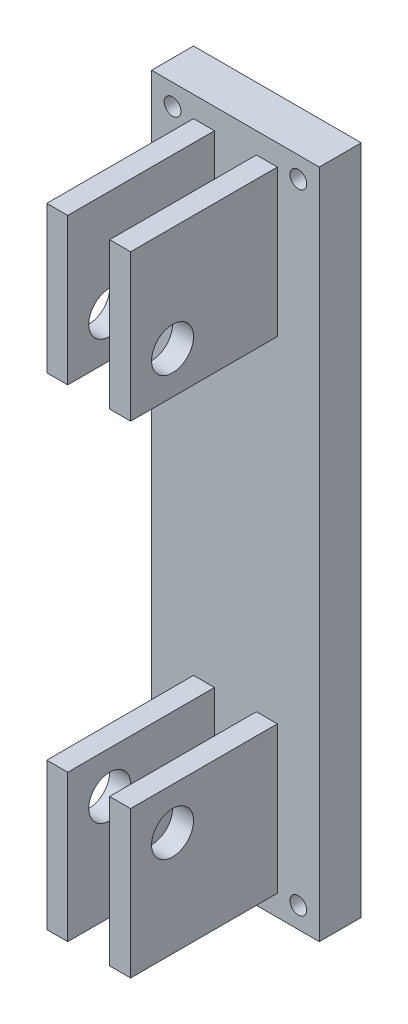
SolidWorks part; units mm, degrees
ref_plane "Front Plane" through (0, 0, 0) normal (0, 0, 1) x (1, 0, 0)
ref_plane "Top Plane" through (0, 0, 0) normal (0, 1, 0) x (1, 0, 0)
ref_plane "Right Plane" through (0, 0, 0) normal (1, 0, 0) x (0, 0, -1)
sketch "Sketch1" plane through (0, 0, 0) normal (0, 0, 1) x (1, 0, 0)
  line L1 (2, -8) -> (-2, -8)
  line L2 (2, -8) -> (2, 8)
  line L3 (2, 8) -> (-2, 8)
  line L4 (-2, -8) -> (-2, 8)
  line L5 (2, -8) -> (-2, 8) construction
  line L6 (2, 8) -> (-2, -8) construction
  point P0 (0, 0)
  dimension "D1" = 4
  dimension "D2" = 16
extrude "Boss-Extrude1" add sketch "Sketch1" along normal blind 1
sketch "Sketch2" plane through (0, 0, 1) normal (0, 0, 1) x (1, 0, 0)
  line L1 (0.5, -7.5) -> (1, -7.5)
  line L2 (0.5, -7.5) -> (0.5, 7.5)
  line L3 (0.5, 7.5) -> (1, 7.5)
  line L4 (1, -7.5) -> (1, 7.5)
  line L5 (0.5, -7.5) -> (1, 7.5) construction
  line L6 (0.5, 7.5) -> (1, -7.5) construction
  line L7 (-0.5, -7.5) -> (-1, -7.5)
  line L8 (-0.5, -7.5) -> (-0.5, 7.5)
  line L9 (-0.5, 7.5) -> (-1, 7.5)
  line L10 (-1, -7.5) -> (-1, 7.5)
  line L11 (-0.5, -7.5) -> (-1, 7.5) construction
  line L12 (-0.5, 7.5) -> (-1, -7.5) construction
  point P0 (0.75, 0)
  point P5 (-0.75, 0)
  dimension "D1" = 0.5
  dimension "D2" = 0.5
  dimension "D3" = 15
  dimension "D5" = 0.5
extrude "Boss-Extrude2" add sketch "Sketch2" along normal blind 3.5
sketch "Sketch3" plane through (-1, 0, 0) normal (-1, 0, 0) x (0, 0, 1)
  line L0 (4.5, 7.5) -> (4.5, -7.5) construction
  circle A0 centre (3.5, 5) radius 0.5
  circle A1 centre (3.5, -5) radius 0.5
  dimension "D1" = 1
  dimension "D2" = 1
  dimension "D3" = 10
  dimension "D4" = 5
extrude "Cut-Extrude1" cut sketch "Sketch3" against normal blind 4.5
sketch "Sketch4" plane through (0, 0, 1) normal (0, 0, 1) x (1, 0, 0)
  line L0 (2, -8) -> (2, 8) construction
  line L1 (-1.5, -7.5) -> (1.5, -7.5) construction
  line L2 (-1.5, -7.5) -> (-1.5, 7.5) construction
  line L3 (-1.5, 7.5) -> (1.5, 7.5) construction
  line L4 (1.5, -7.5) -> (1.5, 7.5) construction
  line L5 (-1.5, -7.5) -> (1.5, 7.5) construction
  line L6 (-1.5, 7.5) -> (1.5, -7.5) construction
  line L7 (2, 8) -> (-2, 8) construction
  circle A0 centre (-1.5, 7.5) radius 0.2
  circle A1 centre (-1.5, -7.5) radius 0.2
  circle A2 centre (1.5, -7.5) radius 0.2
  circle A3 centre (1.5, 7.5) radius 0.2
  point P0 (0, 0)
  dimension "D3" = 0.4
  dimension "D1" = 0.5
  dimension "D2" = 0.5
extrude "Cut-Extrude2" cut sketch "Sketch4" against normal blind 4.5
sketch "Sketch5" plane through (0, 0, 4.5) normal (0, 0, 1) x (1, 0, 0)
  line L1 (-4.0963, -4) -> (4.0963, -4)
  line L2 (-4.0963, -4) -> (-4.0963, 4)
  line L3 (-4.0963, 4) -> (4.0963, 4)
  line L4 (4.0963, -4) -> (4.0963, 4)
  line L5 (-4.0963, -4) -> (4.0963, 4) construction
  line L6 (-4.0963, 4) -> (4.0963, -4) construction
  point P0 (0, 0)
  dimension "D1" = 8
extrude "Cut-Extrude3" cut sketch "Sketch5" against normal up to surface (3.5 mm away) up to face at (1.7, 7.5, 1)
